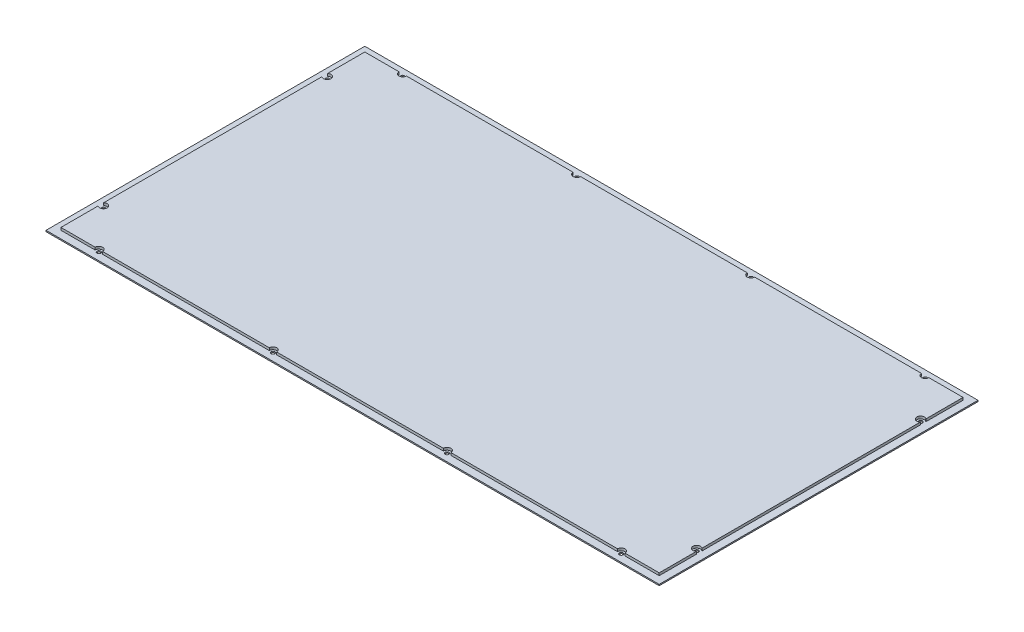
from build123d import *

# Parameters (mm, degrees)
SKETCH1_W           = 493
SKETCH1_H           = 256.3
BOSS_EXTRUDE1_DEPTH = 1.5
SKETCH2_W           = 493
SKETCH2_H           = 256.3
SKETCH2_W_2         = 481
SKETCH2_H_2         = 244.3
CUT_EXTRUDE1_DEPTH  = 2
SKETCH3_R           = 1.5
CUT_EXTRUDE2_DEPTH  = 278.83749297
SKETCH4_R           = 1.5
CUT_EXTRUDE3_DEPTH  = 278.83749297
SKETCH5_R           = 3
CUT_EXTRUDE4_DEPTH  = 2


with BuildPart() as part:
    # Sketch1 → Boss-Extrude1 (new, symmetric)
    with BuildSketch(Plane(origin=(0, 0, 0), x_dir=(1, 0, 0), z_dir=(0, 1, 0))):
        Rectangle(SKETCH1_W, SKETCH1_H)
    extrude(amount=BOSS_EXTRUDE1_DEPTH, both=True)

    # Sketch2 → Cut-Extrude1 (cut)
    with BuildSketch(Plane(origin=(0, 1.5, 0), x_dir=(1, 0, 0), z_dir=(0, 1, 0))):
        Rectangle(SKETCH2_W, SKETCH2_H)
        Rectangle(SKETCH2_W_2, SKETCH2_H_2, mode=Mode.SUBTRACT)
    extrude(amount=-CUT_EXTRUDE1_DEPTH, mode=Mode.SUBTRACT)

    # Sketch3 → Cut-Extrude2 (cut, through all)
    with BuildSketch(Plane(origin=(0, 1.5, 0), x_dir=(1, 0, 0), z_dir=(0, 1, 0))):
        with Locations(Location((-70, 122.15, 0), (0, 0, 270))):
            Circle(SKETCH3_R)
        with Locations(Location((-210, 122.15, 0), (0, 0, 270))):
            Circle(SKETCH3_R)
        with Locations((70, 122.15)):
            Circle(SKETCH3_R)
        with Locations((210, 122.15)):
            Circle(SKETCH3_R)
    cut_extrude2 = extrude(amount=-CUT_EXTRUDE2_DEPTH, mode=Mode.SUBTRACT)

    # Mirror1: Cut-Extrude2 across plane
    add(cut_extrude2.mirror(Plane.XY), mode=Mode.SUBTRACT)

    # Sketch4 → Cut-Extrude3 (cut, through all)
    with BuildSketch(Plane(origin=(0, 1.5, 0), x_dir=(1, 0, 0), z_dir=(0, 1, 0))):
        with Locations(Location((-238.5, 90, 0), (0, 0, 270))):
            Circle(SKETCH4_R)
        with Locations(Location((-238.5, -90, 0), (0, 0, 90))):
            Circle(SKETCH4_R)
    cut_extrude3 = extrude(amount=-CUT_EXTRUDE3_DEPTH, mode=Mode.SUBTRACT)

    # Mirror2: Cut-Extrude3 across plane
    add(cut_extrude3.mirror(Plane(origin=(0, 0, 0), x_dir=(0, 0, 1), z_dir=(1, 0, 0))), mode=Mode.SUBTRACT)

    # Sketch5 → Cut-Extrude4 (cut)
    with BuildSketch(Plane(origin=(0, 1.5, 0), x_dir=(1, 0, 0), z_dir=(0, 1, 0))):
        with Locations((-210, 122.15)):
            Circle(SKETCH5_R)
        with Locations((-70, 122.15)):
            Circle(SKETCH5_R)
        with Locations((70, 122.15)):
            Circle(SKETCH5_R)
        with Locations((210, 122.15)):
            Circle(SKETCH5_R)
        with Locations((238.5, 90)):
            Circle(SKETCH5_R)
        with Locations((238.5, -90)):
            Circle(SKETCH5_R)
        with Locations((210, -122.15)):
            Circle(SKETCH5_R)
        with Locations((70, -122.15)):
            Circle(SKETCH5_R)
        with Locations((-70, -122.15)):
            Circle(SKETCH5_R)
        with Locations((-210, -122.15)):
            Circle(SKETCH5_R)
        with Locations((-238.5, -90)):
            Circle(SKETCH5_R)
        with Locations((-238.5, 90)):
            Circle(SKETCH5_R)
    extrude(amount=-CUT_EXTRUDE4_DEPTH, mode=Mode.SUBTRACT)


solid = part.part
